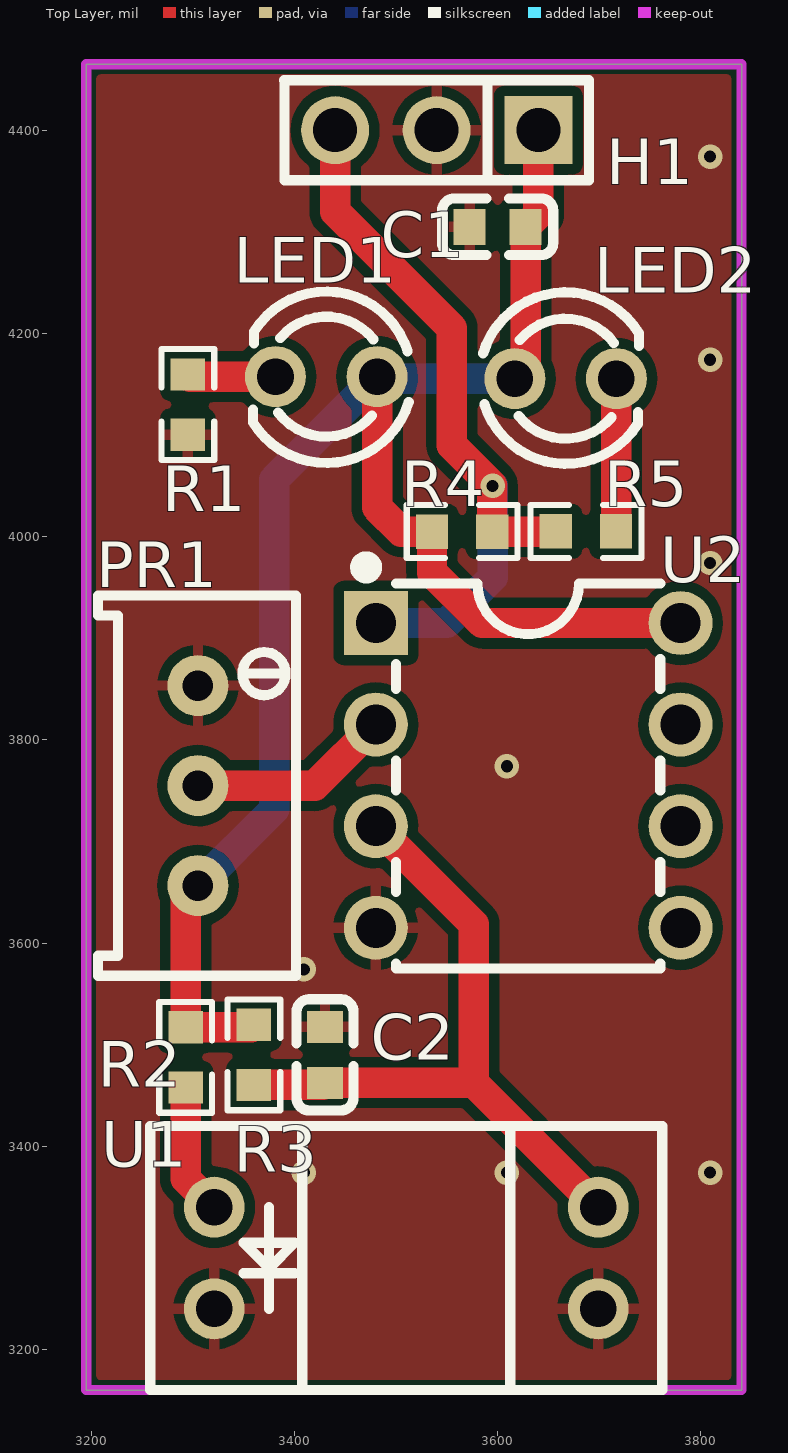
[diagram p0: Top Layer view]
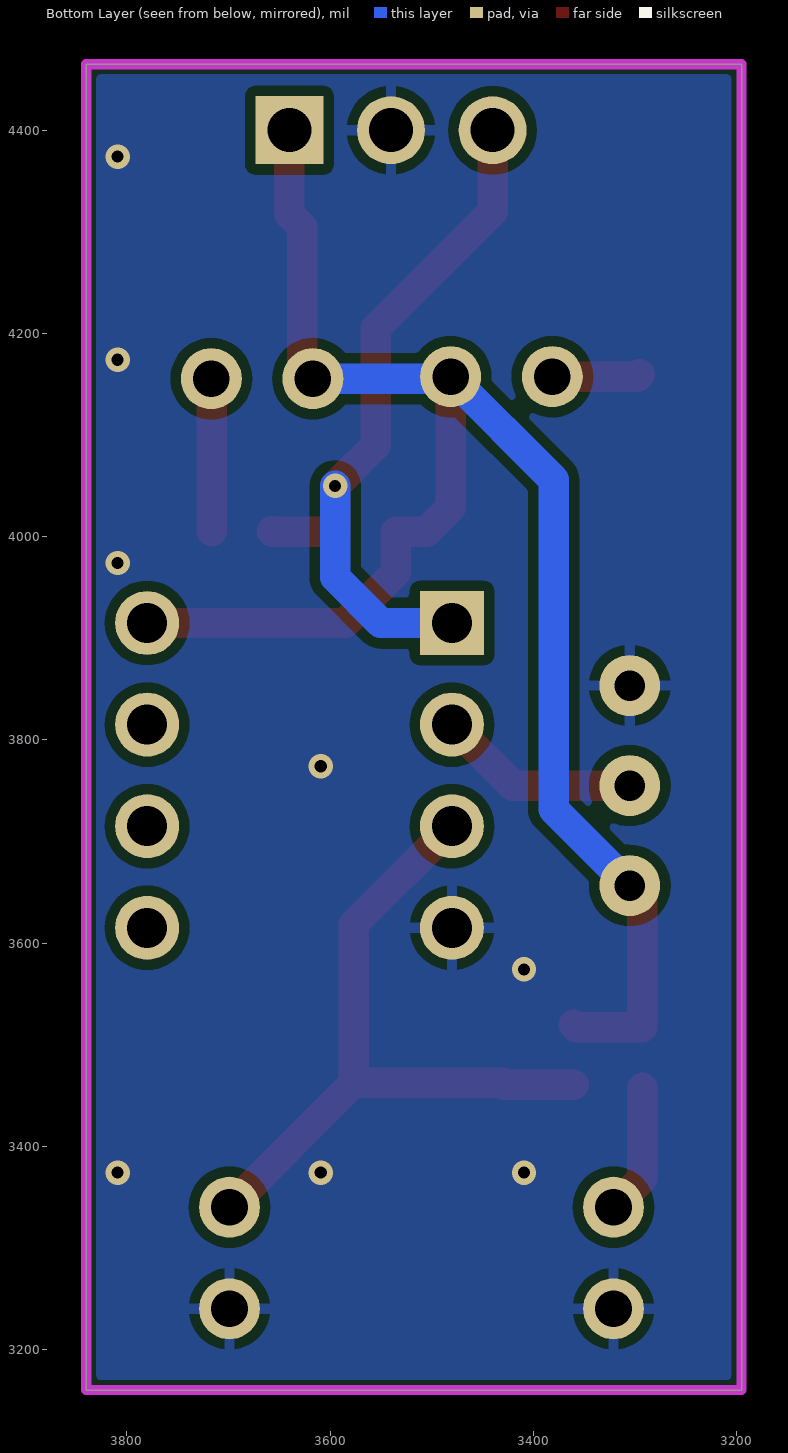
[diagram p1: Bottom Layer view, seen from below]
# Altium PCB MISC51709.pcbdoc
Units mil, origin at the board's own origin, x right, y up, seen from the top; angles counter-clockwise.
Board outline 645 x 1305 mil, 2 copper layers (Top Layer, Bottom Layer), stack 62.206 mil thick; 13 components, 8 nets, 36 pads, 9 vias.

## Layer stack, top to bottom
Top Solder Mask Layer: solder mask 0.394, Dk 3.3
Top Layer: signal copper 1.379
Dielectric1: surface 59.449, FR4, Dk 4.5
Bottom Layer: signal copper 1.378
Bottom Solder Mask Layer: solder mask 0.394, Dk 3.3

## Board outline
3195,4465 3195,3160 3840,3160 3840,4465

## Design rules (kind name [scope] priority, off if disabled: settings)
BoardOutlineClearance copperThickness2oz_1 [All] p2 off: genericclearance=7.99 ignorepadtopadclearanceinfootprint=FALSE except(0: Arc-SplitContinuation Track-SplitContinuation SMDPad-SplitContinuation THPad-SplitContinuation Via-SplitContinuation Fill-SplitContinuation Region-SplitContinuation Poly-SplitContinuation Text-SplitContinuation Hole-SplitContinuation; 5.98: Arc-CutoutEdge SMDPad-CutoutEdge THPad-CutoutEdge Via-CutoutEdge Fill-CutoutEdge Region-CutoutEdge Text-CutoutEdge; 6.93: Hole-OutlineEdge Hole-CutoutEdge; 10: Poly-OutlineEdge Poly-CutoutEdge; 11.81: Arc-OutlineEdge Track-OutlineEdge SMDPad-OutlineEdge THPad-OutlineEdge Via-OutlineEdge Fill-OutlineEdge Region-OutlineEdge Text-OutlineEdge Track-CutoutEdge)
BoardOutlineClearance copperThickness1oz_1 [All] p4: genericclearance=4.02 ignorepadtopadclearanceinfootprint=FALSE except(0: Arc-SplitContinuation Track-SplitContinuation SMDPad-SplitContinuation THPad-SplitContinuation Via-SplitContinuation Fill-SplitContinuation Region-SplitContinuation Poly-SplitContinuation Text-SplitContinuation Hole-SplitContinuation; 6: SMDPad-CutoutEdge THPad-CutoutEdge Via-CutoutEdge Fill-CutoutEdge Region-CutoutEdge Text-CutoutEdge; 6.93: Hole-OutlineEdge Hole-CutoutEdge; 10: Poly-OutlineEdge Poly-CutoutEdge; 11.8: Arc-OutlineEdge Track-OutlineEdge SMDPad-OutlineEdge THPad-OutlineEdge Via-OutlineEdge Fill-OutlineEdge Region-OutlineEdge Text-OutlineEdge; 11.81: Arc-CutoutEdge Track-CutoutEdge)
Clearance copperThickness2oz [All] p1 off: gap=7.99 ignorepadtopadclearanceinfootprint=FALSE except(5.98: SMDPad-Track SMDPad-SMDPad THPad-Track SMDPad-THPad THPad-THPad Track-Via SMDPad-Via THPad-Via Via-Via Fill-Track Region-Track Fill-SMDPad Region-SMDPad Fill-THPad Region-THPad Fill-Via Region-Via Fill-Fill Fill-Region Region-Region Arc-Track Arc-SMDPad Arc-THPad Arc-Via Fill-Arc Region-Arc Arc-Arc Text-Track SMDPad-Text Text-THPad Text-Via Fill-Text Region-Text Arc-Text Text-Text; 6.93: Hole-Track Hole-SMDPad Hole-THPad Hole-Via Fill-Hole Region-Hole Hole-Arc Hole-Text; 10: Poly-Track Poly-SMDPad Poly-THPad Poly-Via Poly-Fill Poly-Region Poly-Poly Poly-Arc Poly-Text Poly-Hole)
Clearance copperThickness1oz [All] p3: gap=4.02 ignorepadtopadclearanceinfootprint=FALSE except(5.98: SMDPad-Track SMDPad-SMDPad THPad-Track SMDPad-THPad THPad-THPad Track-Via SMDPad-Via THPad-Via Via-Via Fill-Track Region-Track Fill-SMDPad Region-SMDPad Fill-THPad Region-THPad Fill-Via Region-Via Fill-Fill Fill-Region Region-Region; 6: Arc-Track Arc-SMDPad Arc-THPad Arc-Via Fill-Arc Region-Arc Arc-Arc Text-Track SMDPad-Text Text-THPad Text-Via Fill-Text Region-Text Arc-Text Text-Text; 6.93: Hole-Track Hole-SMDPad Hole-THPad Hole-Via Fill-Hole Region-Hole Hole-Arc Hole-Text; 10: Poly-Track Poly-SMDPad Poly-THPad Poly-Via Poly-Fill Poly-Region Poly-Poly Poly-Arc Poly-Text Poly-Hole)
DiffPairsRouting differentialPair [All] p1: maxlimit=6 minlimit=6 mostfreqgap=6 toplayer_minwidth=5 toplayer_prefwidth=10 toplayer_maxwidth=100 toplayer_mingap=6 toplayer_prefgap=6 toplayer_maxgap=6 bottomlayer_minwidth=5 bottomlayer_prefwidth=10 bottomlayer_maxwidth=100 bottomlayer_mingap=6 bottomlayer_prefgap=6 bottomlayer_maxgap=6 maxuncoupledlength=10
HoleToHoleClearance otherClearance [All] p1: gap=11.81 allowstackedmicrovias=TRUE
Length netLength [All] p1: minlimit=0 maxlimit=0
MatchedLengths netLengthTolerance [All] p1: tolerance=1000
PasteMaskExpansion pasteMaskExpansion [All] p1: expansion=0
PlaneConnect innerPlane [All] p1: planeconnectstyle=Relief reliefexpansion=20 reliefentries=4 reliefconductorwidth=10 reliefairgap=10
PolygonConnect copperRegion [(InNet('GND'))] p1: connectstyle=Relief reliefconductorwidth=10 reliefentries=4 polygonreliefangle="90 Angle" airgapwidth=10 via.connectstyle=Relief via.reliefconductorwidth=10 via.reliefentries=4 via.polygonreliefangle="90 Angle" via.airgapwidth=10
RoutingVias viaSize [All] p1: holewidth=12.01 width=24.02 viastyle="Through Hole" minholewidth=11.81 minwidth=19.68 maxholewidth=248.03 maxwidth=393.7
SolderMaskExpansion solderMaskExpansion [IsVia] p1: expansion=-1000 istentingtop=TRUE
SolderMaskExpansion solderMaskExpansion [All] p2: expansion=2 istentingtop=FALSE
Width copperThickness2oz_2 [All] p1 off: maxlimit=100 minlimit=8 preferedwidth=10
Width copperThickness1oz_2 [All] p2: maxlimit=100 minlimit=5 preferedwidth=10

## Components (designator, comment, footprint, x,y, rotation, side; value= is the part's Value field where it differs from the comment)
C1 "100nF" C0603 3600,4305 r0 top
C2 "100nF" C0603 3430,3490 r270 top
H1 "" HDR-TH_3P-P2.54-V-M 3540,4400 r180 top
LED1 "" LED_TH-3mm 3431.28,4157.46 r180 top
LED2 "" LED_TH-3mm 3666.87,4155.51 r0 top
PR1 "10kΩ" R_3296 3310,3755 r270 top
R1 "1K" R0603 3295,4130 r90 top
R2 "100" R0603 3292.87,3487.47 r90 top
R3 "10K" R0603 3360,3490 r90 top
R4 "10K" R0603 3565,4005 r180 top
R5 "1K" R0603 3686.87,4005.11 r0 top
U1 "ZOS-T1305-A02(ZD)" OPTO-TH_ZOS-T1305-A02 3510,3290 r0 top
U2 "LM393N-ON" PDIP-8_L9.6-W6.4-P2.54-LS7.9-BL 3630,3765 r270 top

## Footprints (in the part's own frame and the unit in brackets; to place one, negate y for a bottom-side part, rotate by r counter-clockwise, add the part's x,y. Pads: shape width x height; smd on the part's side, far side on the other; paste and mask are expansions set on the pad)
C0603 [mm]
  rect 0.8x0.9 smd: 1(-0.7,0) 2(0.7,0)
  silkscreen extent -1.39,-0.71 1.39,0.71
HDR-TH_3P-P2.54-V-M [mm]
  rect 1.7x1.7 hole 1.1: 1(-2.54,0)
  round 1.7 hole 1.1: 2(0,0) 3(2.54,0)
  silkscreen extent -3.81,-1.25 3.81,1.25
LED_TH-3mm [mil]
  round 60 hole 36 paste+0 mask+2: 1(-50,0) 2(50,0)
  silkscreen extent -81,-84 72,85
OPTO-TH_ZOS-T1305-A02 [mil]
  round 60 hole 36: 1(-188.98,50) 2(-188.98,-50) 3(188.98,-50) 4(188.98,50)
  silkscreen extent -252,-130 252,130
PDIP-8_L9.6-W6.4-P2.54-LS7.9-BL [mil]
  rect 63x63 hole 39.37: 1(-150,-150)
  round 63 hole 39.37: 2(-50,-150) 3(50,-150) 4(150,-150) 5(150,150) 6(50,150) 7(-50,150) 8(-150,150)
  silkscreen extent -213,-167 190,130
R0603 [mil]
  rect 31.75x34.02 smd paste-3937.01 mask+2: 1(-29.66,0) 2(29.66,0)
  silkscreen extent -55,-26 55,26
R_3296 [mil]
  round 60 hole 30 paste+0 mask+2: 1(-98.4,-5) 2(0,-5) 3(98.4,-5)
  silkscreen extent -187,-103 187,92

## Via types
v1: diameter 24.02, hole 12, Top Layer to Bottom Layer, 9 vias

## Nets (pads, with @x,y where several pads share a name; then routed paths per layer and width w, separated by ;. In a path a pad name is that pad's centre, name@x,y a point inside that pad or via, vN(x,y) a via of type N, cw(c..) or ccw(c..) an arc to the next point about the centre after c; other vN are vias at no path point)
$1N2: LED1.2 R1.2 | length 87.2
  Top Layer w30: R1.2 3297.2,4157.46 LED1.2
$1N6: R2.1 U1.1 | length 129.5
  Top Layer w30: R2.1 3292.87,3368.15 U1.1
$1N7: C2.2 R3.1 U1.4 U2.3 | length 683.1
  Top Layer w30: R3.1 3427.9,3460.34 C2.2 3576.54,3462.44 ; U2.3 3576.54,3618.46 3576.54,3462.44 ; U1.4 3576.54,3462.44
$1N8: PR1.2 U2.2 | length 199.9
  Top Layer w30: PR1.2 3420,3755 U2.2
$1N10: LED2.2 R5.2 | length 150.5
  Top Layer w30: R5.2 3716.53,4155.17 LED2.2
DO: H1.3 R4.1 R5.1 U2.1 | length 745.3
  Top Layer w30: H1.3 3440,4320 3555,4205 3555,4090 3594.66,4050.34 R4.1 3657.11,4005 R5.1
  Bottom Layer w30: U2.1 3550,3915 3595,3960 v1(3595,4050)
GND: C1.1 C2.1 H1.2 PR1.1 R1.1 U1.2 U1.3 U2.4
  other v1: 3409.1,3374.1 3609.1,3374.1 3809.1,3374.1 3409.1,3574.1 3609.1,3774.1 3809.1,3974.1 3809.1,4174.1 3809.1,4374.1
VCC: C1.2 H1.1 LED1.1 LED2.1 PR1.3 R2.2 R3.2 R4.2 U2.8 | length 1675.2
  Top Layer w30: PR1.3 3292.87,3644.47 R2.2 3357.47,3517.13 R3.2 ; LED1.1 3481.28,4028.72 3505,4005 R4.2 3535.34,3964.66 3585,3915 U2.8 ; LED2.1 3627.56,4166.2 C1.2 3640,4317.44 H1.1
  Bottom Layer w30: PR1.3 3380,3731.6 3380,4056.18 LED1.1 3483.23,4155.51 LED2.1
pads on no net: U2.5 U2.6 U2.7

## Polygon pours and split planes (outlines as drawn)
GND on Top Layer (solid, remove dead copper, pour order 0): 3000,4590 3000,3000 4020,3000 4020,4590
GND on Bottom Layer (solid, remove dead copper, pour order 2): 3110,4565 3110,3010 3925,3010 3925,4565

## Keep-outs
Board Outline Layer:
  the board outline again, w10